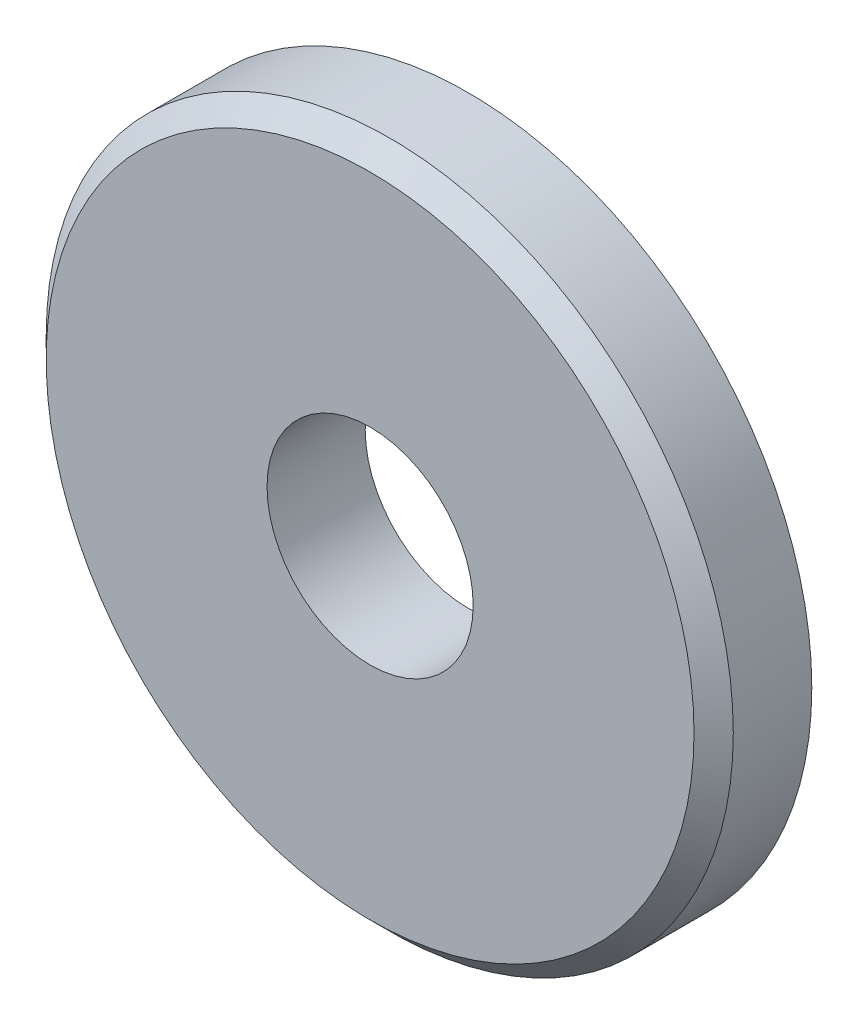
SolidWorks part; units mm, degrees
material "1023 碳钢板 (SS)"
ref_plane "前视基准面" through (0, 0, 0) normal (0, 0, 1) x (1, 0, 0)
ref_plane "上视基准面" through (0, 0, 0) normal (0, 1, 0) x (1, 0, 0)
ref_plane "右视基准面" through (0, 0, 0) normal (1, 0, 0) x (0, 0, -1)
sketch "草图1" plane through (0, 0, 0) normal (0, 0, 1) x (1, 0, 0)
  circle A0 centre (0, 0) radius 17.5
  circle A1 centre (0, 0) radius 5.25
  dimension "D1" = 35
  dimension "D2" = 10.5
extrude "凸台-拉伸1" add sketch "草图1" along normal blind 5
chamfer "倒角1" distance 1 angle 45 1 edges at (17.5, 0, 5)
